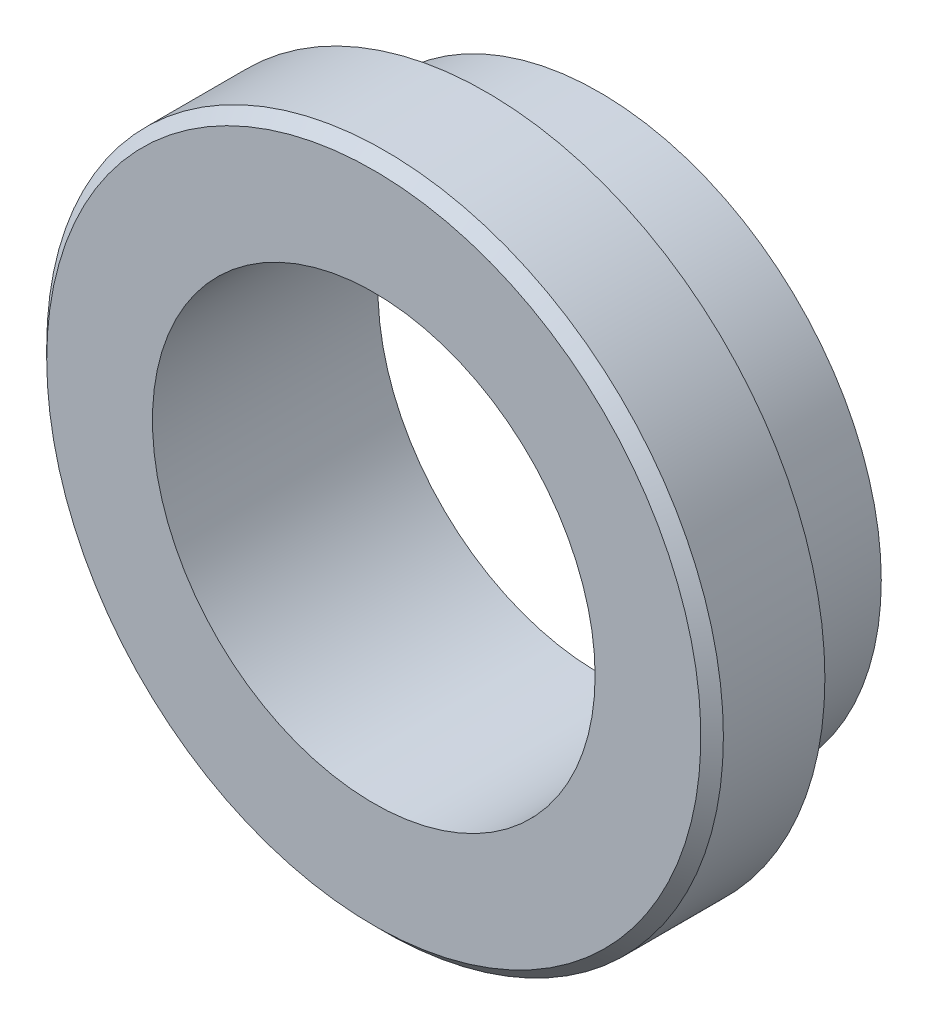
from build123d import *

# Parameters (mm, degrees)
G1_1_4_TAPPED_HOLE1_D = 39.25
CHAMFER1_SIZE         = 1


with BuildPart() as part:
    # Sketch1 → Revolve1 (revolve)
    with BuildSketch(Plane(origin=(0, 0, 0), x_dir=(0, 0, -1), z_dir=(1, 0, 0)), mode=Mode.PRIVATE) as revolve1_sk:
        Polygon((0, 0), (0, 25), (-10, 25), (-10, 30), (-20, 30), (-20, 0), align=None)
    revolve(revolve1_sk.sketch.rotate(Axis((0, 0, 20), (0, 0, -1)), 90), axis=Axis((0, 0, 20), (0, 0, -1)))

    # G1-1/4 Tapped Hole1 (through all)
    with Locations(Plane.XY.offset(20)):
        with Locations((0, 0)):
            Hole(G1_1_4_TAPPED_HOLE1_D / 2)

    # Chamfer1
    chamfer1_edges = [part.edges().sort_by_distance(p)[0] for p in [
        (-30, 0, 20),
    ]]
    chamfer(chamfer1_edges, length=CHAMFER1_SIZE)


solid = part.part
